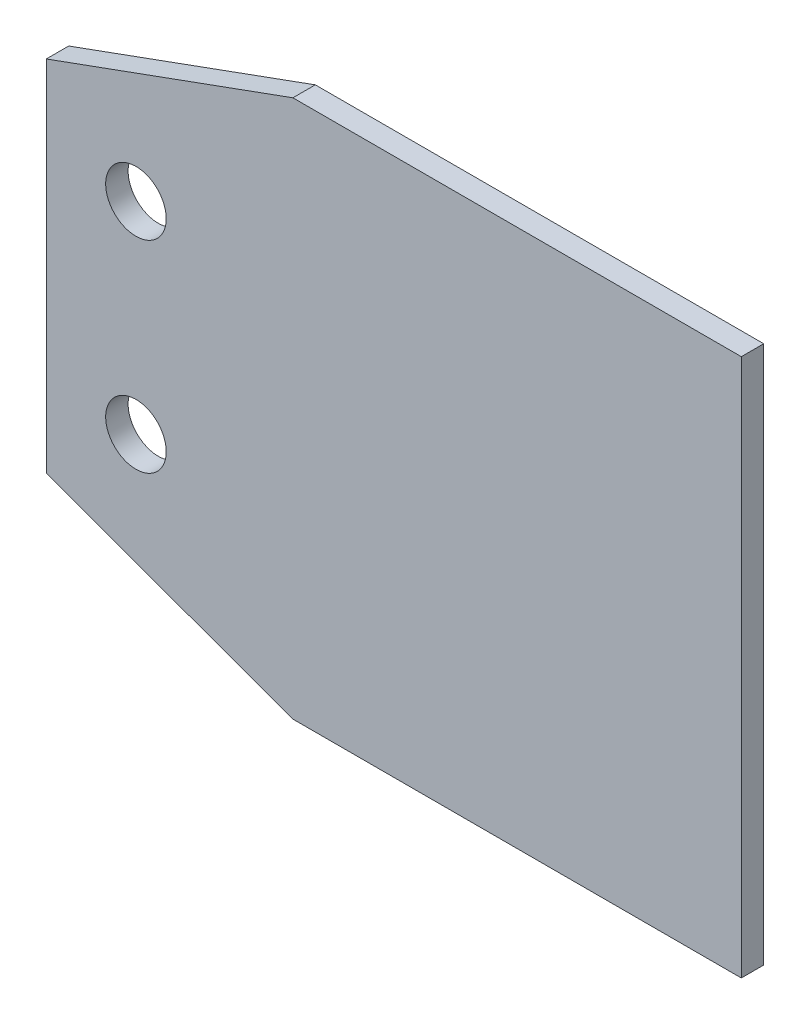
from build123d import *

# Parameters (mm, degrees)
SKETCH_1_W          = 310
SKETCH_1_H          = 240
EXTRUDE_1_DEPTH     = 10
SKETCH_2_R          = 13.5
CUT_EXTRUDE_1_DEPTH = 10


with BuildPart() as part:
    # 草图1 → 凸台-拉伸1 (new body)
    with BuildSketch(Plane.XY):
        Rectangle(SKETCH_1_W, SKETCH_1_H)
    extrude(amount=EXTRUDE_1_DEPTH)

    # 草图2 → 切除-拉伸1 (cut)
    with BuildSketch(Plane.XY.offset(10)):
        with Locations((-115, -45)):
            Circle(SKETCH_2_R)
        with Locations((-115, 45)):
            Circle(SKETCH_2_R)
        Polygon((-155, -80), (-45, -120), (-155, -120), align=None)
        Polygon((-155, 80), (-45, 120), (-155, 120), align=None)
    extrude(amount=-CUT_EXTRUDE_1_DEPTH, mode=Mode.SUBTRACT)


solid = part.part
